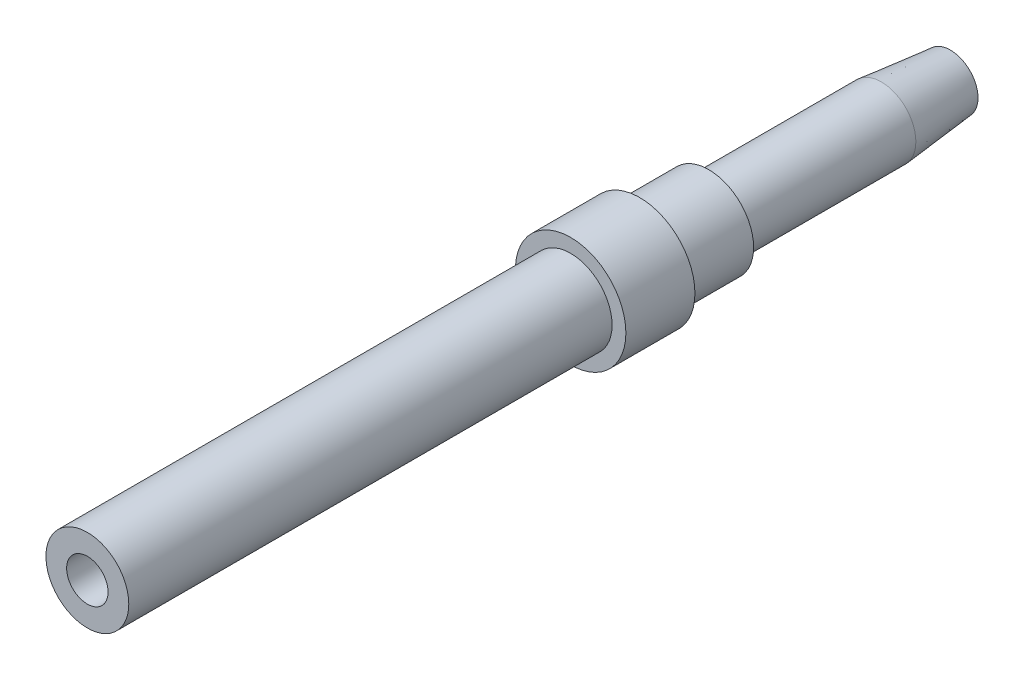
SolidWorks part; units mm, degrees
material "45#"
ref_plane "Front Plane" through (0, 0, 0) normal (0, 0, 1) x (1, 0, 0)
ref_plane "Top Plane" through (0, 0, 0) normal (0, 1, 0) x (1, 0, 0)
ref_plane "Right Plane" through (0, 0, 0) normal (1, 0, 0) x (0, 0, -1)
sketch "Sketch1" plane through (0, 0, 0) normal (0, 0, 1) x (1, 0, 0)
  circle A0 centre (0, 0) radius 5
  circle A1 centre (0, 0) radius 3
  dimension "D1" = 6
  dimension "D2" = 10
extrude "Boss-Extrude1" add sketch "Sketch1" along normal blind 35
sketch "Sketch2" plane through (0, 0, 35) normal (0, 0, 1) x (1, 0, 0)
  circle A0 centre (0, 0) radius 6.5
  circle A1 centre (0, 0) radius 3
  dimension "D1" = 13
  dimension "D2" = 6
extrude "Boss-Extrude2" add sketch "Sketch2" along normal blind 10
sketch "Sketch3" plane through (0, 0, 45) normal (0, 0, 1) x (1, 0, 0)
  circle A0 centre (0, 0) radius 8
  circle A1 centre (0, 0) radius 3
  dimension "D1" = 16
  dimension "D2" = 6
extrude "Boss-Extrude3" add sketch "Sketch3" along normal blind 10
sketch "Sketch4" plane through (0, 0, 55) normal (0, 0, 1) x (1, 0, 0)
  circle A0 centre (0, 0) radius 3
  circle A1 centre (0, 0) radius 6
  dimension "D1" = 6
  dimension "D2" = 12
extrude "Boss-Extrude4" add sketch "Sketch4" along normal blind 70
chamfer "Chamfer1" distance 1 distance2 10 1 edges at (5, 0, 0)
